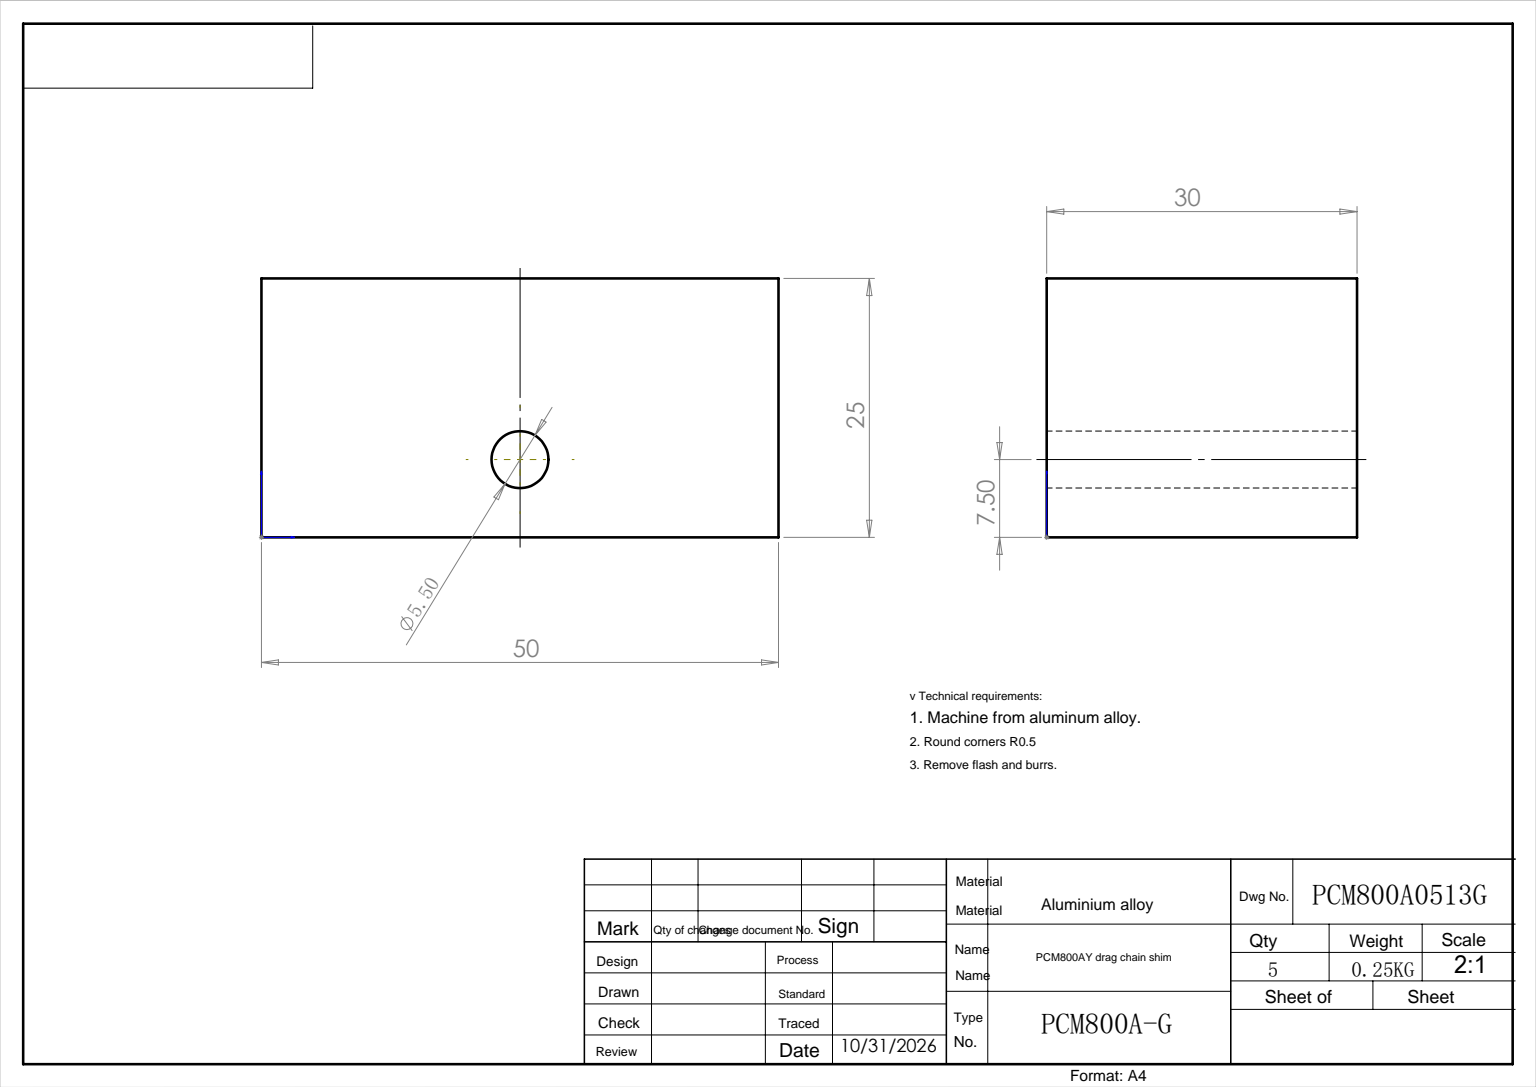
SolidWorks part; units mm, degrees
ref_plane "前视基准面" through (0, 0, 0) normal (0, 0, 1) x (1, 0, 0)
ref_plane "上视基准面" through (0, 0, 0) normal (0, 1, 0) x (1, 0, 0)
ref_plane "右视基准面" through (0, 0, 0) normal (1, 0, 0) x (0, 0, -1)
sketch "草图1" plane through (0, 0, 0) normal (0, 0, 1) x (1, 0, 0)
  line L1 (0, 0) -> (50, 0)
  line L2 (0, 0) -> (0, 25)
  line L3 (0, 25) -> (50, 25)
  line L4 (50, 0) -> (50, 25)
  dimension "D1" = 25
  dimension "D2" = 50
extrude "凸台-拉伸1" add sketch "草图1" along normal blind 30
sketch "草图2" plane through (0, 0, 30) normal (0, 0, 1) x (1, 0, 0)
  line L0 (25, 0) -> (25, 33.9068) construction
  line L1 (0, 0) -> (50, 0) construction
  circle A0 centre (25, 7.5) radius 2.75
  dimension "D1" = 5.5
  dimension "D2" = 7.5
extrude "切除-拉伸1" cut sketch "草图2" against normal blind 37
